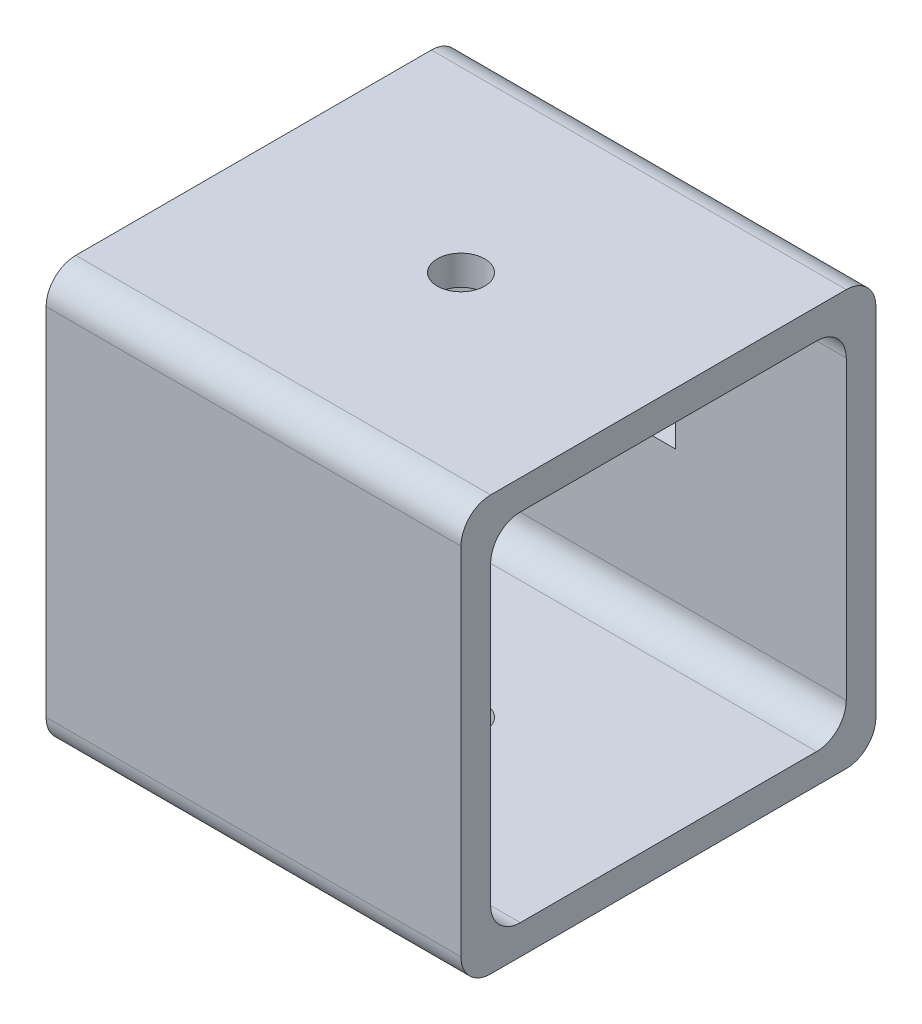
from build123d import *

# Parameters (mm, degrees)
SKETCH1_W           = 70
SKETCH1_H           = 70
BOSS_EXTRUDE1_DEPTH = 70
SKETCH2_W           = 60
SKETCH2_H           = 60
CUT_EXTRUDE1_DEPTH  = 104
SKETCH3_W           = 12.4
SKETCH3_H           = 5.4
CUT_EXTRUDE2_DEPTH  = 10
SKETCH4_R           = 4
CUT_EXTRUDE3_DEPTH  = 122
FILLET1_R           = 5


with BuildPart() as part:
    # Sketch1 → Boss-Extrude1 (new body)
    with BuildSketch(Plane.XY):
        Rectangle(SKETCH1_W, SKETCH1_H)
    extrude(amount=BOSS_EXTRUDE1_DEPTH)

    # Sketch2 → Cut-Extrude1 (cut)
    with BuildSketch(Plane(origin=(35, 0, 0), x_dir=(0, 0, -1), z_dir=(1, 0, 0))):
        with Locations((-35, 0)):
            Rectangle(SKETCH2_W, SKETCH2_H)
    extrude(amount=-CUT_EXTRUDE1_DEPTH, mode=Mode.SUBTRACT)

    # Sketch3 → Cut-Extrude2 (cut)
    with BuildSketch(Plane(origin=(0, 0, 0), x_dir=(-1, 0, 0), z_dir=(0, 0, -1))):
        Rectangle(SKETCH3_W, SKETCH3_H)
    extrude(amount=-CUT_EXTRUDE2_DEPTH, mode=Mode.SUBTRACT)

    # Sketch4 → Cut-Extrude3 (cut)
    with BuildSketch(Plane.XZ.offset(35)):
        with Locations(Location((0, 35, 0), (0, 0, 270))):
            Circle(SKETCH4_R)
    extrude(amount=-CUT_EXTRUDE3_DEPTH, mode=Mode.SUBTRACT)

    # Fillet1
    fillet1_edges = [part.edges().sort_by_distance(p)[0] for p in [
        (0, 35, 70),
        (0, -30, 5),
        (0, -30, 65),
        (0, 30, 65),
        (0, 30, 5),
        (0, 35, 0),
        (0, -35, 0),
        (0, -35, 70),
    ]]
    fillet(fillet1_edges, radius=FILLET1_R)


solid = part.part
